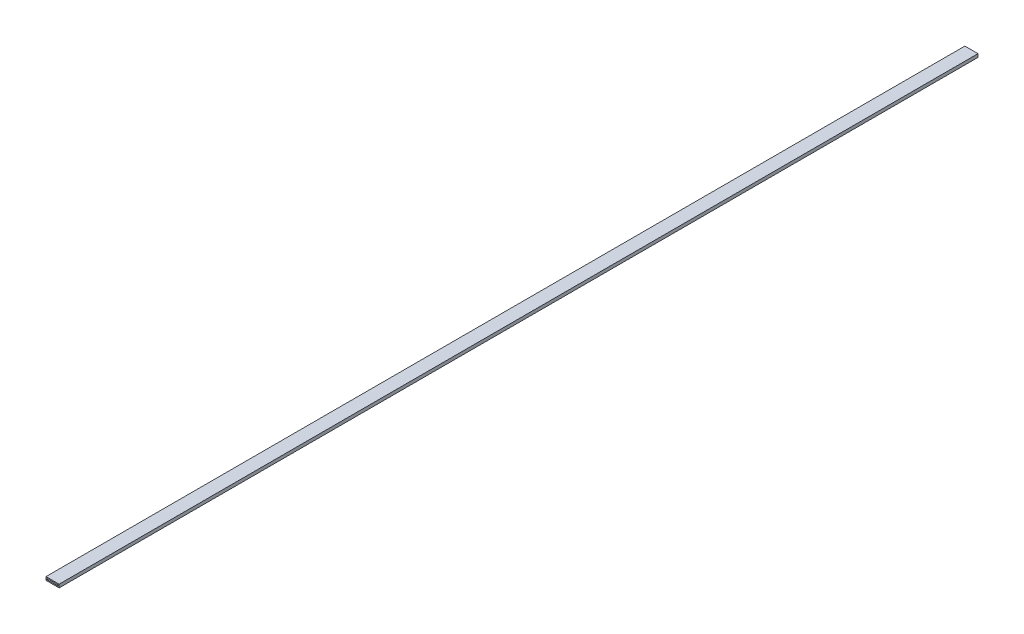
from build123d import *

# Parameters (mm, degrees)
SKETCH1_W           = 12
SKETCH1_H           = 3
BOSS_EXTRUDE1_DEPTH = 840
SKETCH2_W           = 10
SKETCH2_H           = 1
CUT_EXTRUDE1_DEPTH  = 841.951655259


with BuildPart() as part:
    # Sketch1 → Boss-Extrude1 (new body)
    with BuildSketch(Plane.XY):
        with Locations((-25.901003365, 22.624934563)):
            Rectangle(SKETCH1_W, SKETCH1_H)
    extrude(amount=BOSS_EXTRUDE1_DEPTH)

    # Sketch2 → Cut-Extrude1 (cut, through all)
    with BuildSketch(Plane.XY.offset(840)):
        with Locations((-25.901003365, 22.624934563)):
            Rectangle(SKETCH2_W, SKETCH2_H)
    extrude(amount=-CUT_EXTRUDE1_DEPTH, mode=Mode.SUBTRACT)


solid = part.part
